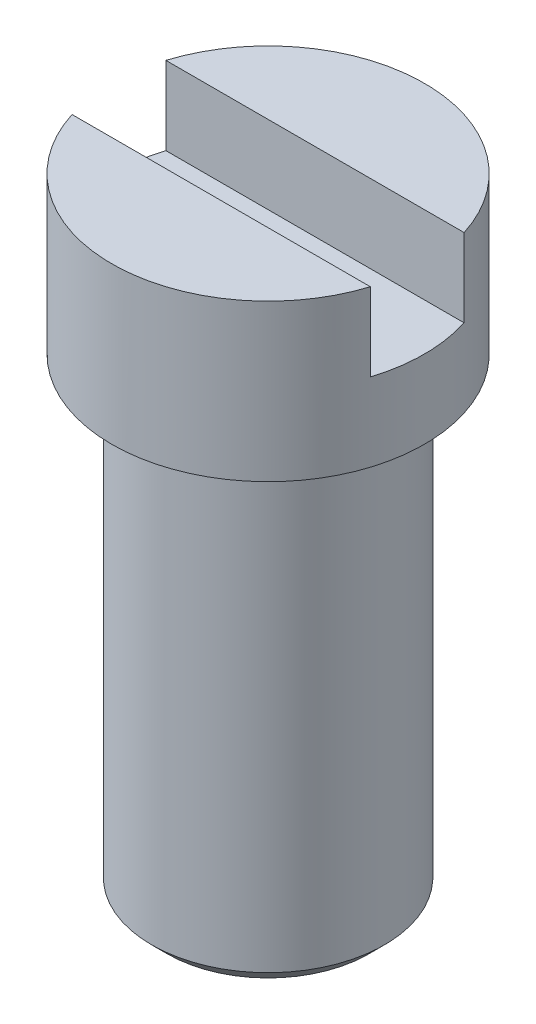
SolidWorks part; units mm, degrees
ref_plane "前视基准面" through (0, 0, 0) normal (0, 0, 1) x (1, 0, 0)
ref_plane "上视基准面" through (0, 0, 0) normal (0, 1, 0) x (1, 0, 0)
ref_plane "右视基准面" through (0, 0, 0) normal (1, 0, 0) x (0, 0, -1)
other "Configuration Table"
sketch "草图1" plane through (0, 0, 0) normal (0, 1, 0) x (1, 0, 0)
  circle A0 centre (0, 0) radius 7.45
  dimension "D1" = 14.9
extrude "凸台-拉伸1" add sketch "草图1" against normal blind 30 contours A0
sketch "草图2" plane through (0, 0, 0) normal (0, 1, 0) x (1, 0, 0)
  circle A0 centre (0, 0) radius 10
  dimension "D1" = 20
extrude "凸台-拉伸2" add sketch "草图2" along normal blind 10 contours A0
sketch "草图4" plane through (0, 10, 0) normal (0, 1, 0) x (1, 0, 0)
  line L1 (-25, -3) -> (25, -3)
  line L2 (-25, -3) -> (-25, 3)
  line L3 (-25, 3) -> (25, 3)
  line L4 (25, -3) -> (25, 3)
  line L5 (-25, -3) -> (25, 3) construction
  line L6 (-25, 3) -> (25, -3) construction
  point P0 (0, 0)
  dimension "D1" = 50
  dimension "D2" = 6
extrude "切除-拉伸2" cut sketch "草图4" against normal blind 5 contours L1 L4 L3 L2
chamfer "倒角1" distance 1 angle 45 1 edges at (0, -30, 7.45)
